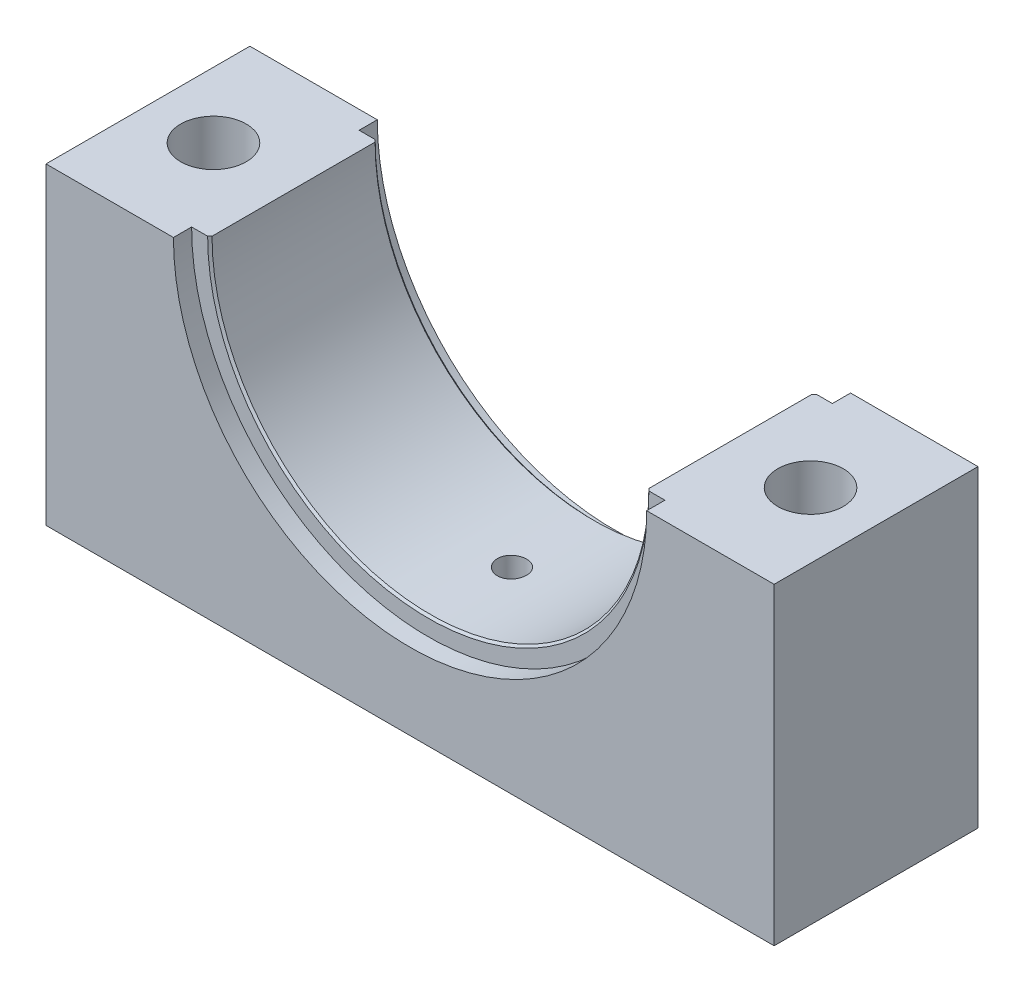
SolidWorks part; units mm, degrees
material "Q235-A"
ref_plane "Front Plane" through (0, 0, 0) normal (0, 0, 1) x (1, 0, 0)
ref_plane "Top Plane" through (0, 0, 0) normal (0, 1, 0) x (1, 0, 0)
ref_plane "Right Plane" through (0, 0, 0) normal (1, 0, 0) x (0, 0, -1)
sketch "Sketch1" plane through (0, 0, 0) normal (0, 0, 1) x (1, 0, 0)
  line L0 (-50, 0) -> (-30, 0)
  line L1 (-50, -43) -> (50, -43)
  line L2 (-50, -43) -> (-50, 0)
  line L4 (50, -43) -> (50, 0)
  line L5 (-50, -43) -> (0, 0) construction
  line L6 (22.7456, -19.5612) -> (50, -43) construction
  line L7 (30, 0) -> (50, 0)
  arc A0 (-30, 0) -> (30, 0) centre (0, 0) ccw
  point P0 (0, 0)
  dimension "D1" = 43
  dimension "D2" = 100
extrude "Boss-Extrude1" add sketch "Sketch1" along normal blind 28
sketch "Sketch2" plane through (0, 0, 28) normal (0, 0, 1) x (1, 0, 0)
  circle A0 centre (0, 0) radius 32.5
extrude "Cut-Extrude1" cut sketch "Sketch2" against normal blind 2.5
sketch "Sketch3" plane through (0, 0, 0) normal (0, 0, -1) x (-1, 0, 0)
  circle A1 centre (0, 0) radius 32.5
  circle A2 centre (0, 0) radius 32.5
  dimension "D1" = 0
extrude "Cut-Extrude2" cut sketch "Sketch3" against normal blind 2.5
chamfer "Chamfer1" distance 0.3 angle 45 2 edges at (0, -30, 2.5) (0, -30, 25.5)
sketch "Sketch4" plane through (0, 0, 0) normal (0, 1, 0) x (1, 0, 0)
  line L0 (-41, -14) -> (41, -14)
  line L1 (-50, -28) -> (-50, 0) construction
  line L4 (50, -28) -> (50, 0) construction
  point P6 (50, -14)
  dimension "D1" = 82
  dimension "D2" = 9
  dimension "D3" = 0
hole_wizard "Hole1" positions "Sketch5" profile "Sketch6" legacy end condition through all
sketch "Sketch5" plane through (0, 0, 0) normal (0, 1, 0) x (1, 0, 0)
  point P0 (-41, -14)
  point P3 (41, -14)
sketch "Sketch6" plane through (-41, 0, 14) normal (1, 0, 0) x (0, 0, 1)
  line L0 (0, 0) -> (0, 43)
  line L1 (0, 43) -> (4.5, 43)
  line L2 (4.5, 43) -> (4.5, 0)
  line L3 (4.5, 0) -> (0, 0)
  line L4 (0, 110) -> (0, -10) construction
  dimension "直径" = 9
  dimension "深度" = 43
sketch "Sketch8" plane through (0, 0, 0) normal (0, 1, 0) x (1, 0, 0)
  line L0 (0, -28) -> (0, 0)
  line L1 (-32.5, -28) -> (32.5, -28) construction
  line L2 (32.5, 0) -> (-32.5, 0) construction
hole_wizard "Hole2" positions "Sketch9" profile "Sketch10" legacy
sketch "Sketch9" plane through (0, 0, 0) normal (0, 1, 0) x (1, 0, 0)
  line L0 (0, -28) -> (0, 0) construction
  point P0 (0, -14)
sketch "Sketch10" plane through (0, 0, 14) normal (1, 0, 0) x (0, 0, 1)
  line L0 (0, 0) -> (0, 34)
  line L1 (0, 34) -> (2, 34)
  line L2 (2, 34) -> (2, 0)
  line L3 (2, 0) -> (0, 0)
  line L4 (0, 110) -> (0, -10) construction
  dimension "直径" = 4
  dimension "深度" = 34
